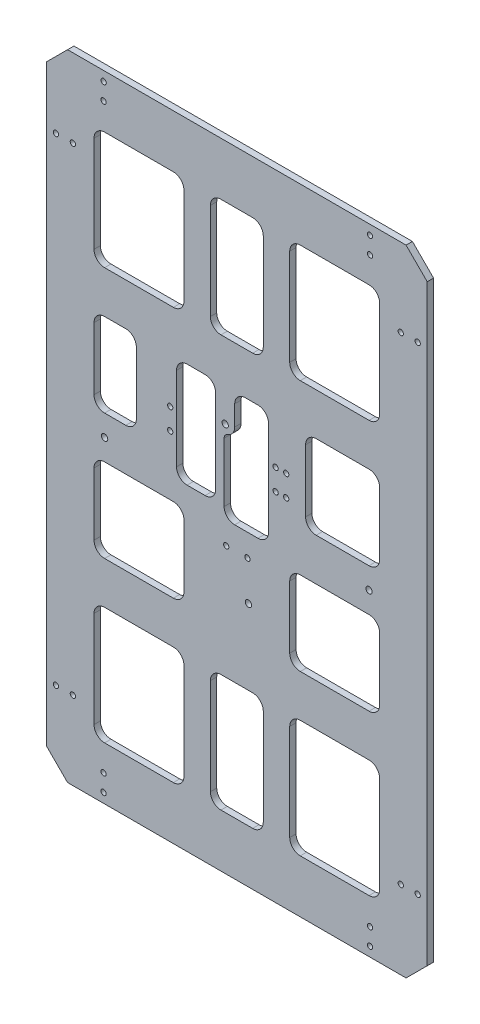
from build123d import *

# Parameters (mm, degrees)
SKETCH_1_R      = 2.5
SKETCH_1_R_2    = 3
EXTRUDE_1_DEPTH = 6


with BuildPart() as part:
    # 草图1 → 凸台-拉伸1 (new body)
    with BuildSketch(Plane(origin=(0, 0, 0), x_dir=(-1, 0, 0), z_dir=(0, 0, -1))):
        Polygon((160, -300), (180, -280), (180, 280), (160, 300), (-160, 300), (-180, 280), (-180, -280), (-160, -300), align=None)
        with Locations(Location((-36.672939041, 56.4, 0), (0, 0, 180))):
            Circle(SKETCH_1_R, mode=Mode.SUBTRACT)
        with Locations(Location((-10, -31.172939041, 0), (0, 0, 180))):
            Circle(SKETCH_1_R, mode=Mode.SUBTRACT)
        with Locations(Location((10, -31.172939041, 0), (0, 0, 180))):
            Circle(SKETCH_1_R, mode=Mode.SUBTRACT)
        with Locations(Location((-171, 225.965949669, 0), (0, 0, 180))):
            Circle(SKETCH_1_R, mode=Mode.SUBTRACT)
        with Locations(Location((-155, 225.965949669, 0), (0, 0, 180))):
            Circle(SKETCH_1_R, mode=Mode.SUBTRACT)
        with Locations(Location((-125.965949669, 275, 0), (0, 0, 180))):
            Circle(SKETCH_1_R, mode=Mode.SUBTRACT)
        with Locations(Location((-125.899824793, 291, 0), (0, 0, 180))):
            Circle(SKETCH_1_R, mode=Mode.SUBTRACT)
        with Locations(Location((-171, -225.902192547, 0), (0, 0, 180))):
            Circle(SKETCH_1_R, mode=Mode.SUBTRACT)
        with Locations(Location((-155, -225.902192547, 0), (0, 0, 180))):
            Circle(SKETCH_1_R, mode=Mode.SUBTRACT)
        with Locations(Location((-125.965949669, -275.000477451, 0), (0, 0, 180))):
            Circle(SKETCH_1_R, mode=Mode.SUBTRACT)
        with Locations(Location((-125.965949669, -291.000477451, 0), (0, 0, 180))):
            Circle(SKETCH_1_R, mode=Mode.SUBTRACT)
        with Locations(Location((125.899824793, 291, 0), (0, 0, 180))):
            Circle(SKETCH_1_R, mode=Mode.SUBTRACT)
        with Locations(Location((125.965949669, 275, 0), (0, 0, 180))):
            Circle(SKETCH_1_R, mode=Mode.SUBTRACT)
        with Locations(Location((171, 225.965949669, 0), (0, 0, 180))):
            Circle(SKETCH_1_R, mode=Mode.SUBTRACT)
        with Locations(Location((155, 225.965949669, 0), (0, 0, 180))):
            Circle(SKETCH_1_R, mode=Mode.SUBTRACT)
        with Locations(Location((171, -225.902192547, 0), (0, 0, 180))):
            Circle(SKETCH_1_R, mode=Mode.SUBTRACT)
        with Locations(Location((155, -225.902192547, 0), (0, 0, 180))):
            Circle(SKETCH_1_R, mode=Mode.SUBTRACT)
        with Locations(Location((125.965949669, -291.000477451, 0), (0, 0, 180))):
            Circle(SKETCH_1_R, mode=Mode.SUBTRACT)
        with Locations(Location((125.965949669, -275.000477451, 0), (0, 0, 180))):
            Circle(SKETCH_1_R, mode=Mode.SUBTRACT)
        with Locations(Location((63, 56.4, 0), (0, 0, 180))):
            Circle(SKETCH_1_R, mode=Mode.SUBTRACT)
        with Locations(Location((63, 36.4, 0), (0, 0, 180))):
            Circle(SKETCH_1_R, mode=Mode.SUBTRACT)
        with Locations(Location((-46.672939041, 56.4, 0), (0, 0, 180))):
            Circle(SKETCH_1_R, mode=Mode.SUBTRACT)
        with Locations(Location((-46.672939041, 36.4, 0), (0, 0, 180))):
            Circle(SKETCH_1_R, mode=Mode.SUBTRACT)
        with Locations(Location((-11, -68, 0), (0, 0, 180))):
            Circle(SKETCH_1_R_2, mode=Mode.SUBTRACT)
        with Locations(Location((11, 68, 0), (0, 0, 180))):
            Circle(SKETCH_1_R_2, mode=Mode.SUBTRACT)
        with Locations(Location((-125, 0, 0), (0, 0, 180))):
            Circle(SKETCH_1_R_2, mode=Mode.SUBTRACT)
        with Locations(Location((125, 0, 0), (0, 0, 180))):
            Circle(SKETCH_1_R_2, mode=Mode.SUBTRACT)
        with Locations(Location((-36.672939041, 36.4, 0), (0, 0, 180))):
            Circle(SKETCH_1_R, mode=Mode.SUBTRACT)
        with BuildLine():
            Line((20, 10), (20, 89.042978952))
            ThreePointArc((20, 89.042978952), (22.928932188, 96.114046764), (30, 99.042978952))
            Line((30, 99.042978952), (47, 99.042978952))
            ThreePointArc((47, 99.042978952), (54.071067812, 96.114046764), (57, 89.042978952))
            Line((57, 89.042978952), (57, 10))
            ThreePointArc((57, 10), (54.071067812, 2.928932188), (47, 0))
            Line((47, 0), (30, 0))
            ThreePointArc((30, 0), (22.928932188, 2.928932188), (20, 10))
        make_face(mode=Mode.SUBTRACT)
        with BuildLine():
            Line((2, -10), (-20, -10))
            ThreePointArc((-20, -10), (-27.071067812, -7.071067812), (-30, 0))
            Line((-30, 0), (-30, 89.042978952))
            ThreePointArc((-30, 89.042978952), (-27.071067812, 96.114046764), (-20, 99.042978952))
            Line((-20, 99.042978952), (-8, 99.042978952))
            ThreePointArc((-8, 99.042978952), (-0.928932188, 96.114046764), (2, 89.042978952))
            Line((2, 89.042978952), (2, 70.042978952))
            ThreePointArc((2, 70.042978952), (3.835034191, 64.26947626), (8.666666667, 60.614888536))
            ThreePointArc((8.666666667, 60.614888536), (11.082482905, 58.787594674), (12, 55.900843328))
            Line((12, 55.900843328), (12, 0))
            ThreePointArc((12, 0), (9.071067812, -7.071067812), (2, -10))
        make_face(mode=Mode.SUBTRACT)
        with BuildLine():
            Line((95, 30), (95, 89.042978952))
            ThreePointArc((95, 89.042978952), (97.928932188, 96.114046764), (105, 99.042978952))
            Line((105, 99.042978952), (125, 99.042978952))
            ThreePointArc((125, 99.042978952), (132.071067812, 96.114046764), (135, 89.042978952))
            Line((135, 89.042978952), (135, 30))
            ThreePointArc((135, 30), (132.071067812, 22.928932188), (125, 20))
            Line((125, 20), (105, 20))
            ThreePointArc((105, 20), (97.928932188, 22.928932188), (95, 30))
        make_face(mode=Mode.SUBTRACT)
        with BuildLine():
            Line((125, -250), (60, -250))
            ThreePointArc((60, -250), (52.928932188, -247.071067812), (50, -240))
            Line((50, -240), (50, -149.042978952))
            ThreePointArc((50, -149.042978952), (52.928932188, -141.97191114), (60, -139.042978952))
            Line((60, -139.042978952), (125, -139.042978952))
            ThreePointArc((125, -139.042978952), (132.071067812, -141.97191114), (135, -149.042978952))
            Line((135, -149.042978952), (135, -240))
            ThreePointArc((135, -240), (132.071067812, -247.071067812), (125, -250))
        make_face(mode=Mode.SUBTRACT)
        with BuildLine():
            Line((50, 149.042978952), (50, 240))
            ThreePointArc((50, 240), (52.928932188, 247.071067812), (60, 250))
            Line((60, 250), (125, 250))
            ThreePointArc((125, 250), (132.071067812, 247.071067812), (135, 240))
            Line((135, 240), (135, 149.042978952))
            ThreePointArc((135, 149.042978952), (132.071067812, 141.97191114), (125, 139.042978952))
            Line((125, 139.042978952), (60, 139.042978952))
            ThreePointArc((60, 139.042978952), (52.928932188, 141.97191114), (50, 149.042978952))
        make_face(mode=Mode.SUBTRACT)
        with BuildLine():
            Line((15, 139.042978952), (-15, 139.042978952))
            ThreePointArc((-15, 139.042978952), (-22.071067812, 141.97191114), (-25, 149.042978952))
            Line((-25, 149.042978952), (-25, 240))
            ThreePointArc((-25, 240), (-22.071067812, 247.071067812), (-15, 250))
            Line((-15, 250), (15, 250))
            ThreePointArc((15, 250), (22.071067812, 247.071067812), (25, 240))
            Line((25, 240), (25, 149.042978952))
            ThreePointArc((25, 149.042978952), (22.071067812, 141.97191114), (15, 139.042978952))
        make_face(mode=Mode.SUBTRACT)
        with BuildLine():
            Line((-15, -139.042978952), (15, -139.042978952))
            ThreePointArc((15, -139.042978952), (22.071067812, -141.97191114), (25, -149.042978952))
            Line((25, -149.042978952), (25, -240))
            ThreePointArc((25, -240), (22.071067812, -247.071067812), (15, -250))
            Line((15, -250), (-15, -250))
            ThreePointArc((-15, -250), (-22.071067812, -247.071067812), (-25, -240))
            Line((-25, -240), (-25, -149.042978952))
            ThreePointArc((-25, -149.042978952), (-22.071067812, -141.97191114), (-15, -139.042978952))
        make_face(mode=Mode.SUBTRACT)
        with BuildLine():
            Line((-50, -30), (-50, -89.042978952))
            ThreePointArc((-50, -89.042978952), (-52.928932188, -96.114046764), (-60, -99.042978952))
            Line((-60, -99.042978952), (-125, -99.042978952))
            ThreePointArc((-125, -99.042978952), (-132.071067812, -96.114046764), (-135, -89.042978952))
            Line((-135, -89.042978952), (-135, -30))
            ThreePointArc((-135, -30), (-132.071067812, -22.928932188), (-125, -20))
            Line((-125, -20), (-60, -20))
            ThreePointArc((-60, -20), (-52.928932188, -22.928932188), (-50, -30))
        make_face(mode=Mode.SUBTRACT)
        with BuildLine():
            Line((-50, -149.042978952), (-50, -240))
            ThreePointArc((-50, -240), (-52.928932188, -247.071067812), (-60, -250))
            Line((-60, -250), (-125, -250))
            ThreePointArc((-125, -250), (-132.071067812, -247.071067812), (-135, -240))
            Line((-135, -240), (-135, -149.042978952))
            ThreePointArc((-135, -149.042978952), (-132.071067812, -141.97191114), (-125, -139.042978952))
            Line((-125, -139.042978952), (-60, -139.042978952))
            ThreePointArc((-60, -139.042978952), (-52.928932188, -141.97191114), (-50, -149.042978952))
        make_face(mode=Mode.SUBTRACT)
        with BuildLine():
            Line((-75, 20), (-125, 20))
            ThreePointArc((-125, 20), (-132.071067812, 22.928932188), (-135, 30))
            Line((-135, 30), (-135, 89.042978952))
            ThreePointArc((-135, 89.042978952), (-132.071067812, 96.114046764), (-125, 99.042978952))
            Line((-125, 99.042978952), (-75, 99.042978952))
            ThreePointArc((-75, 99.042978952), (-67.928932188, 96.114046764), (-65, 89.042978952))
            Line((-65, 89.042978952), (-65, 30))
            ThreePointArc((-65, 30), (-67.928932188, 22.928932188), (-75, 20))
        make_face(mode=Mode.SUBTRACT)
        with BuildLine():
            Line((60, -20), (125, -20))
            ThreePointArc((125, -20), (132.071067812, -22.928932188), (135, -30))
            Line((135, -30), (135, -89.042978952))
            ThreePointArc((135, -89.042978952), (132.071067812, -96.114046764), (125, -99.042978952))
            Line((125, -99.042978952), (60, -99.042978952))
            ThreePointArc((60, -99.042978952), (52.928932188, -96.114046764), (50, -89.042978952))
            Line((50, -89.042978952), (50, -30))
            ThreePointArc((50, -30), (52.928932188, -22.928932188), (60, -20))
        make_face(mode=Mode.SUBTRACT)
        with BuildLine():
            Line((-125, 250), (-60, 250))
            ThreePointArc((-60, 250), (-52.928932188, 247.071067812), (-50, 240))
            Line((-50, 240), (-50, 149.042978952))
            ThreePointArc((-50, 149.042978952), (-52.928932188, 141.97191114), (-60, 139.042978952))
            Line((-60, 139.042978952), (-125, 139.042978952))
            ThreePointArc((-125, 139.042978952), (-132.071067812, 141.97191114), (-135, 149.042978952))
            Line((-135, 149.042978952), (-135, 240))
            ThreePointArc((-135, 240), (-132.071067812, 247.071067812), (-125, 250))
        make_face(mode=Mode.SUBTRACT)
    extrude(amount=-EXTRUDE_1_DEPTH)


solid = part.part
